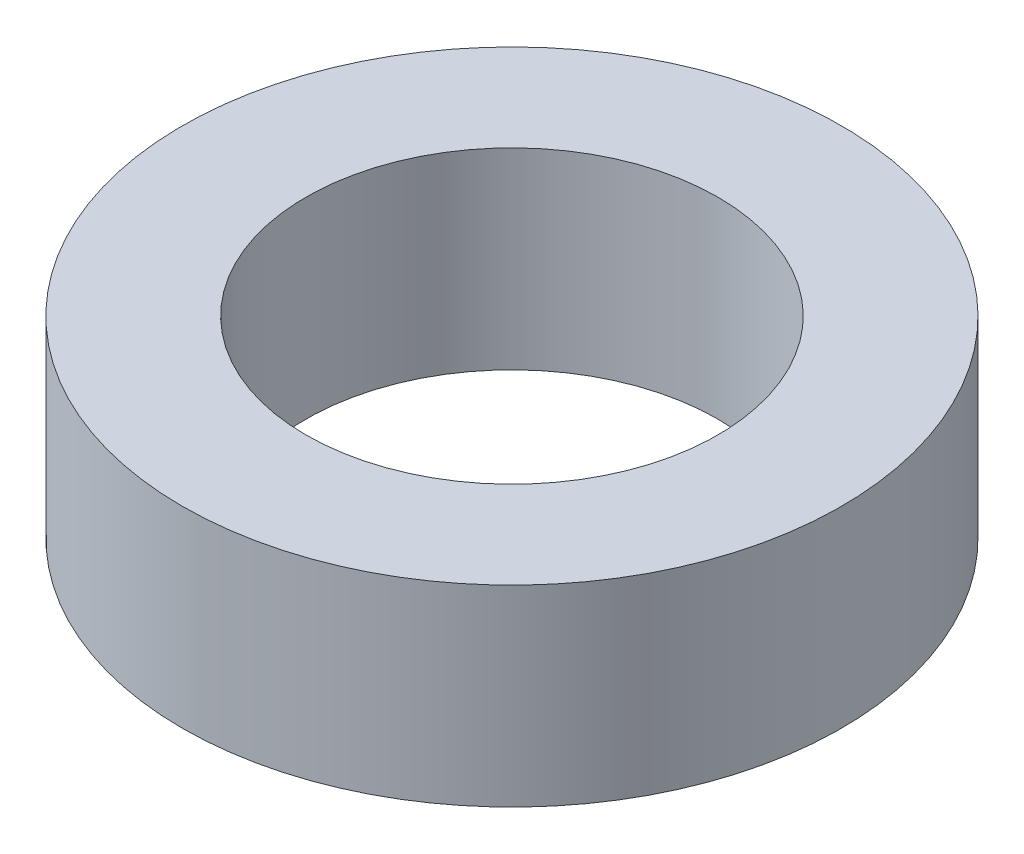
SolidWorks part; units mm, degrees
ref_plane "Front Plane" through (0, 0, 0) normal (0, 0, 1) x (1, 0, 0)
ref_plane "Top Plane" through (0, 0, 0) normal (0, 1, 0) x (1, 0, 0)
ref_plane "Right Plane" through (0, 0, 0) normal (1, 0, 0) x (0, 0, -1)
sketch "Sketch2" plane through (0, 0, 0) normal (0, 1, 0) x (1, 0, 0)
  circle A0 centre (0, 0) radius 12
  circle A1 centre (0, 0) radius 7.5
  dimension "D1" = 15
  dimension "D2" = 24
extrude "Boss-Extrude1" add sketch "Sketch2" along normal blind 7
